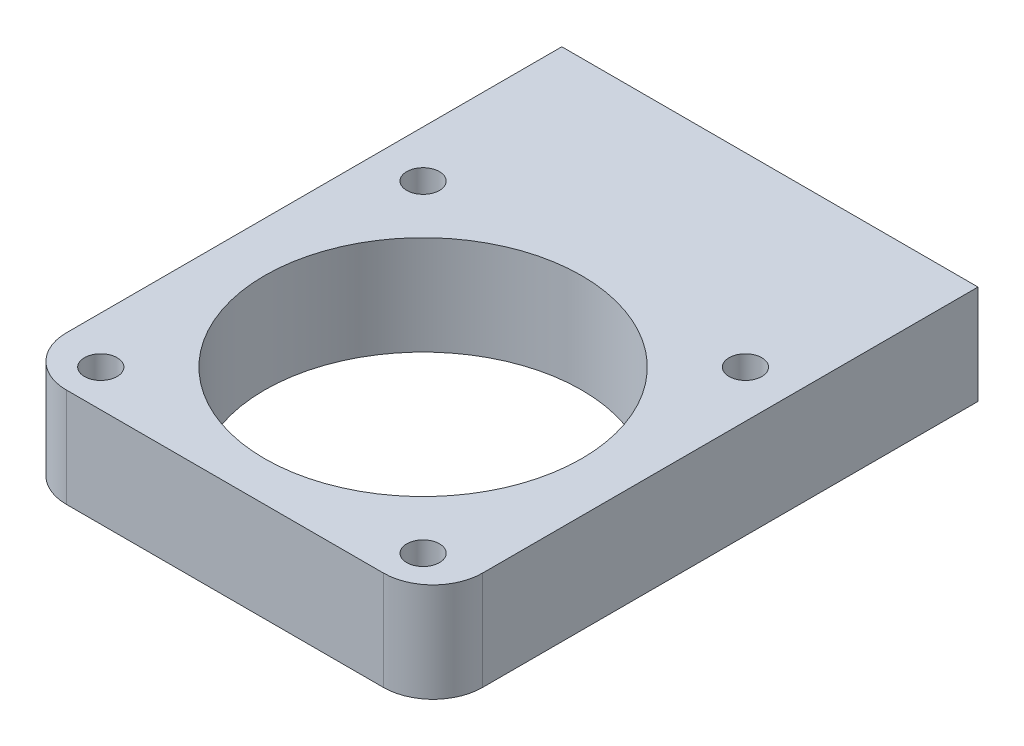
from build123d import *

# Parameters (mm, degrees)
SKETCH_1_W             = 42
SKETCH_1_H             = 72
EXTRUDE_1_DEPTH        = 5
HOLE_WIZARD_M4_2_D     = 3.3
HOLE_WIZARD_M4_2_DEPTH = 12
HOLE_WIZARD_M4_2_TIP   = 0.991420021
SKETCH_6_R             = 16
CUT_EXTRUDE_1_DEPTH    = 43.860237983
CHAMFER_2_SIZE         = 10
FILLET_1_R             = 5
SKETCH_15_W            = 77.686914385
SKETCH_15_H            = 52.90814048
CUT_EXTRUDE_3_DEPTH    = 31
FILLET_2_R             = 5
HOLE_WIZARD_M4_1_D     = 3.3


with BuildPart() as part:
    # 草图1 → 凸台-拉伸1 (new, symmetric)
    with BuildSketch(Plane(origin=(0, 0, 0), x_dir=(1, 0, 0), z_dir=(0, 1, 0))):
        Rectangle(SKETCH_1_W, SKETCH_1_H)
    extrude(amount=EXTRUDE_1_DEPTH, both=True)

    # M4 螺纹孔2
    with Locations(Plane(origin=(0, 0, -36), x_dir=(-1, 0, 0), z_dir=(0, 0, -1))):
        with Locations((-15, 0), (15, 0)):
            Hole(HOLE_WIZARD_M4_2_D / 2, depth=HOLE_WIZARD_M4_2_DEPTH)
            with Locations((0, 0, -(HOLE_WIZARD_M4_2_DEPTH + HOLE_WIZARD_M4_2_TIP / 2))):  # 118° drill point
                Cone(0, HOLE_WIZARD_M4_2_D / 2, HOLE_WIZARD_M4_2_TIP, mode=Mode.SUBTRACT)

    # 草图6 → 切除-拉伸1 (cut, through all)
    with BuildSketch(Plane(origin=(0, 5, 0), x_dir=(1, 0, 0), z_dir=(0, 1, 0))):
        with Locations(Location((0, 1, 0), (0, 0, 270))):
            Circle(SKETCH_6_R)
    extrude(amount=-CUT_EXTRUDE_1_DEPTH, mode=Mode.SUBTRACT)

    # 倒角2
    chamfer_2_edges = [part.edges().sort_by_distance(p)[0] for p in [
        (21, 0, 36),
        (-21, 0, 36),
    ]]
    chamfer(chamfer_2_edges, length=CHAMFER_2_SIZE)

    # 圆角1
    fillet_1_edges = [part.edges().sort_by_distance(p)[0] for p in [
        (11, 0, 36),
        (-11, 0, 36),
        (-21, 0, 26),
        (21, 0, 26),
    ]]
    fillet(fillet_1_edges, radius=FILLET_1_R)

    # 草图15 → 切除-拉伸3 (cut)
    with BuildSketch(Plane(origin=(0, 5, 0), x_dir=(1, 0, 0), z_dir=(0, 1, 0))):
        with Locations((6.233739535, -45.45407024)):
            Rectangle(SKETCH_15_W, SKETCH_15_H)
    extrude(amount=-CUT_EXTRUDE_3_DEPTH, mode=Mode.SUBTRACT)

    # 圆角2
    fillet_2_edges = [part.edges().sort_by_distance(p)[0] for p in [
        (21, 0, 19),
        (-21, 0, 19),
    ]]
    fillet(fillet_2_edges, radius=FILLET_2_R)

    # M4 螺纹孔1 (through all)
    with Locations(Plane(origin=(0, 5, 0), x_dir=(1, 0, 0), z_dir=(0, 1, 0))):
        with Locations((-16.265, 17.265), (16.265, 17.265), (-16.265, -15.265), (16.265, -15.265)):
            Hole(HOLE_WIZARD_M4_1_D / 2)


solid = part.part
